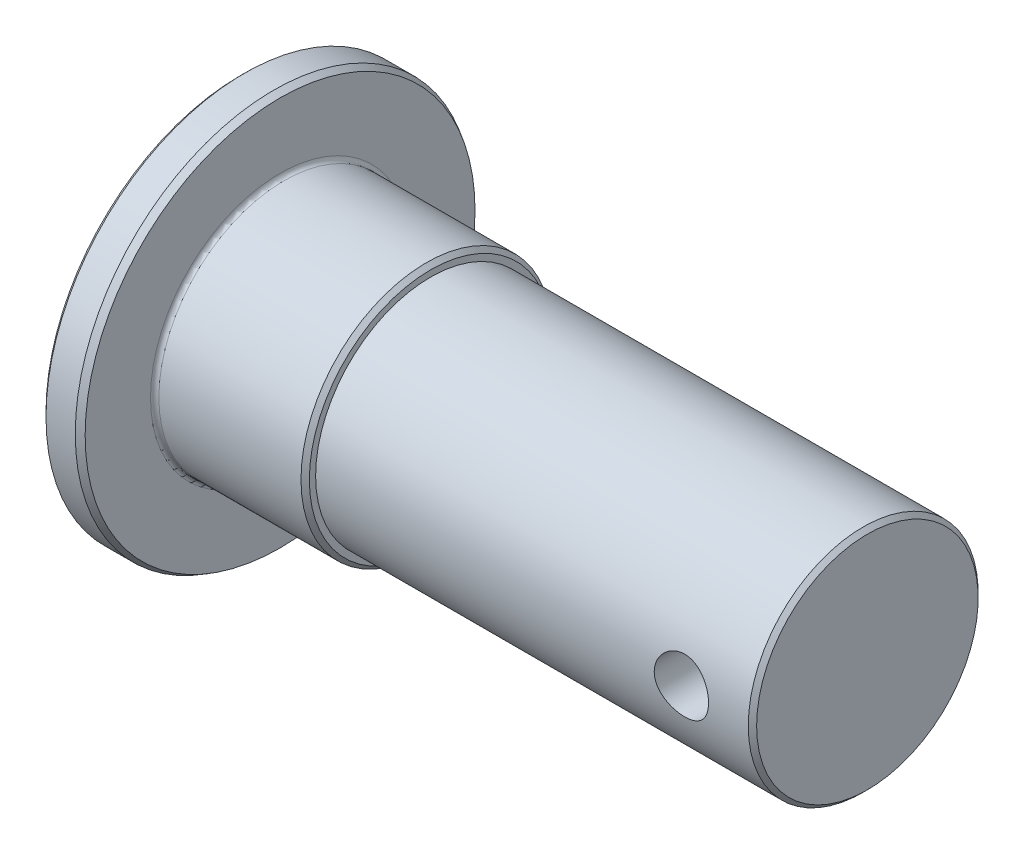
from build123d import *

# Parameters (mm, degrees)
FILLET1_R               = 1
CHAMFER1_SIZE           = 1
CUT_EXTRUDE1_DEPTH      = 165.354799139
CUT_EXTRUDE1_DEPTH_BACK = 165.354799139
SKETCH2_R               = 6.5


with BuildPart() as part:
    # Sketch1 → Revolve1 (revolve)
    with BuildSketch(Plane.XY, mode=Mode.PRIVATE) as revolve1_sk:
        Polygon((0, 0), (0, 47.5), (8, 47.5), (9.5, 46.633974596), (9.5, 30), (45.5, 30), (45.5, 27.5), (150, 27.5), (150, 0), align=None)
    revolve(revolve1_sk.sketch.rotate(Axis((0, 0, 0), (1, 0, 0)), 90), axis=Axis((0, 0, 0), (1, 0, 0)))

    # Fillet1
    fillet1_edges = [part.edges().sort_by_distance(p)[0] for p in [
        (9.5, 0, -30),
    ]]
    fillet(fillet1_edges, radius=FILLET1_R)

    # Chamfer1
    chamfer1_edges = [part.edges().sort_by_distance(p)[0] for p in [
        (150, 0, -27.5),
        (45.5, 0, -30),
        (0, 0, -47.5),
    ]]
    chamfer(chamfer1_edges, length=CHAMFER1_SIZE)

    # Sketch2 → Cut-Extrude1 (cut, two sides: drawn at the far end of the back side and taken through both)
    with BuildSketch(Plane.XY.offset(-CUT_EXTRUDE1_DEPTH_BACK)):
        with Locations((133, 0)):
            Circle(SKETCH2_R)
    extrude(amount=CUT_EXTRUDE1_DEPTH + CUT_EXTRUDE1_DEPTH_BACK, mode=Mode.SUBTRACT)


solid = part.part
